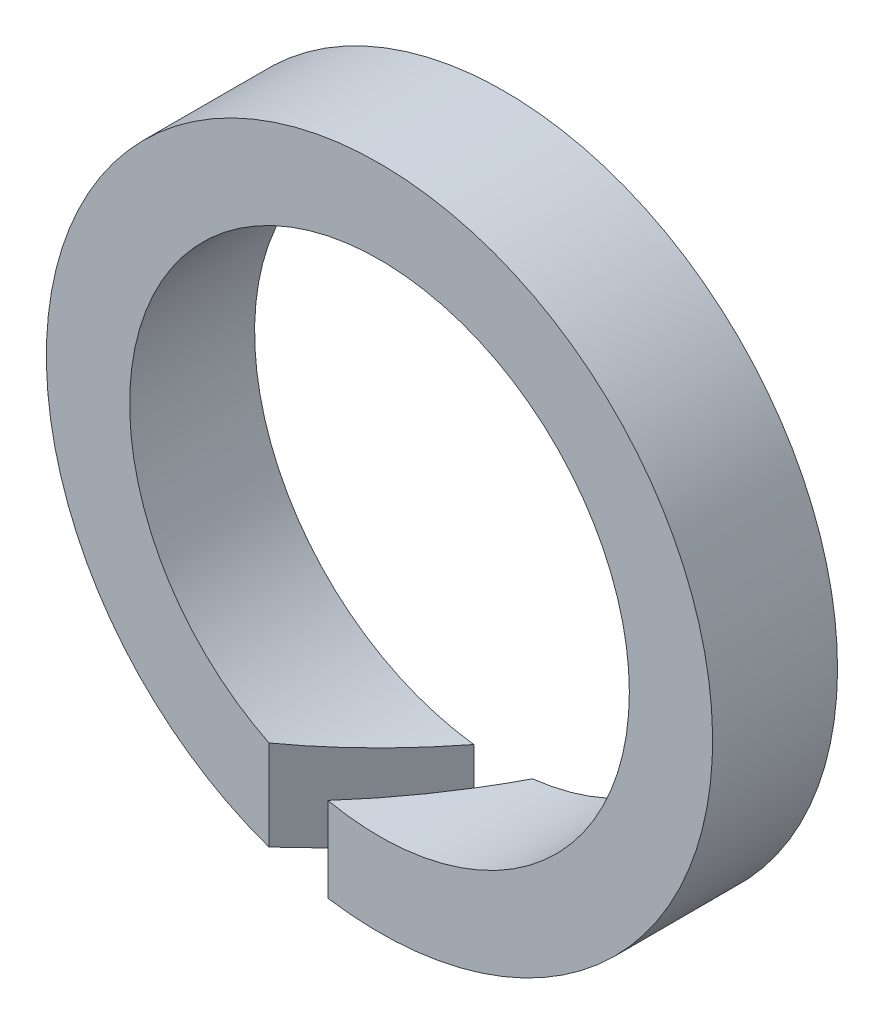
SolidWorks part; units mm, degrees
ref_plane "Front" through (0, 0, 0) normal (0, 0, 1) x (1, 0, 0)
ref_plane "Top" through (0, 0, 0) normal (0, 1, 0) x (1, 0, 0)
ref_plane "Right" through (0, 0, 0) normal (1, 0, 0) x (0, 0, -1)
sketch "Sketch1" plane through (0, 0, 0) normal (0, 1, 0) x (1, 0, 0)
  line L0 (0, 0) -> (0, 20.2398) construction
  line L1 (6, 4.0647) -> (8, 4.0647)
  line L2 (6, 4.0647) -> (6, 7.0647)
  line L3 (6, 7.0647) -> (8, 7.0647)
  line L4 (8, 4.0647) -> (8, 7.0647)
  dimension "D1" = 2
  dimension "D2" = 3
  dimension "D3" = 8
revolve "Revolve1" add sketch "Sketch1" angle 360 about L0
sketch "Sketch2" plane through (0, 0, 0) normal (0, 1, 0) x (1, 0, 0)
  line L0 (-3.2759, 3.0924) -> (2.3796, 11.931)
  line L1 (2.3796, 11.931) -> (3.3821, 11.2896)
  line L2 (3.3821, 11.2896) -> (-2.2734, 2.451)
  line L3 (-2.2734, 2.451) -> (-3.2759, 3.0924)
extrude "Cut-Extrude1" cut sketch "Sketch2" against normal blind 23
